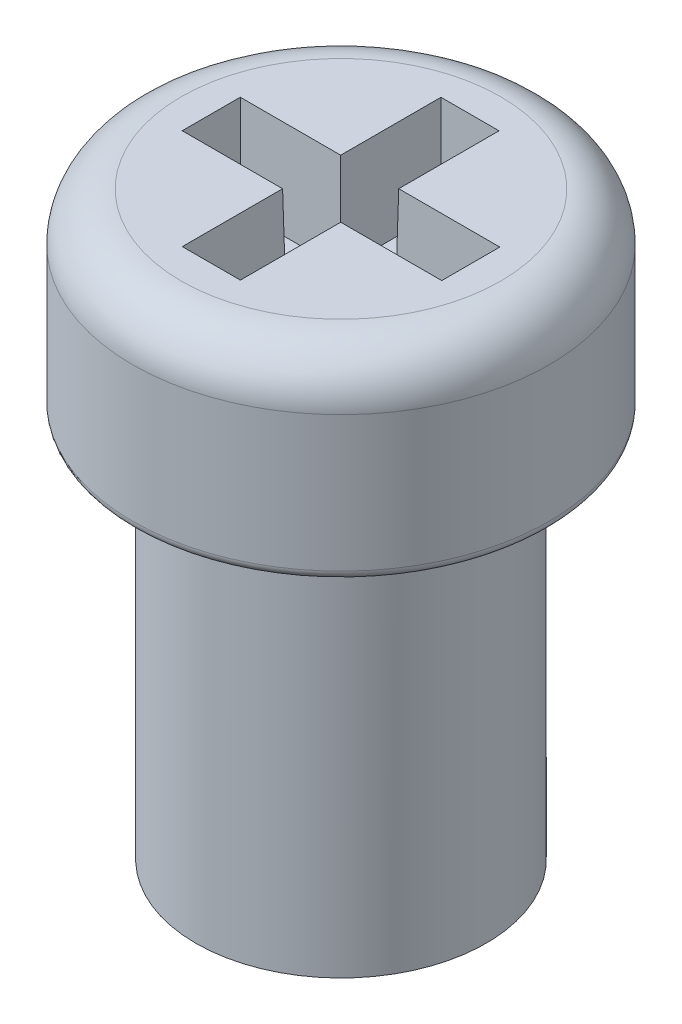
SolidWorks part; units mm, degrees
ref_plane "Front Plane" through (0, 0, 0) normal (0, 0, 1) x (1, 0, 0)
ref_plane "Top Plane" through (0, 0, 0) normal (0, 1, 0) x (1, 0, 0)
ref_plane "Right Plane" through (0, 0, 0) normal (1, 0, 0) x (0, 0, -1)
sketch "Sketch1" plane through (0, 0, 0) normal (0, 1, 0) x (1, 0, 0)
  circle A0 centre (0, 0) radius 2.15
  dimension "D1" = 4.3
extrude "Boss-Extrude1" add sketch "Sketch1" along normal blind 2
sketch "Sketch2" plane through (0, 0, 0) normal (0, -1, 0) x (1, 0, 0)
  circle A0 centre (0, 0) radius 1.5
  dimension "D1" = 3
extrude "Boss-Extrude2" add sketch "Sketch2" along normal blind 4
fillet "Fillet1" radius 0.5 1 edges at (0, 2, 2.15)
fillet "Fillet2" radius 0.1 1 edges at (0, 0, 2.15)
sketch "Sketch3" plane through (0, 2, 0) normal (0, 1, 0) x (1, 0, 0)
  line L0 (0.2966, 0.3) -> (1.3407, 0.3)
  line L1 (-1.3407, -0.3) -> (-0.3034, -0.3)
  line L2 (-1.3407, -0.3) -> (-1.3407, 0.3)
  line L3 (-1.3407, 0.3) -> (-0.3034, 0.3)
  line L4 (1.3407, -0.3) -> (1.3407, 0.3)
  line L5 (0.2966, 0.3) -> (0.2966, 1.3361)
  line L6 (-1.3472, 0.3015) -> (-1.3407, 0.3) construction
  line L7 (-0.3034, -1.3361) -> (0.2966, -1.3361)
  line L8 (-0.3034, -1.3361) -> (-0.3034, -0.3)
  line L9 (-0.3034, 1.3361) -> (0.2966, 1.3361)
  line L10 (0.2966, -1.3361) -> (0.2966, -0.3)
  line L11 (-0.0036, -0.0008) -> (-0.0033, 0.0007) construction
  line L12 (-0.0033, 0.0007) -> (-0.003, -0.0007) construction
  line L13 (-0.3034, 0.3) -> (-0.3034, 1.3361)
  line L15 (0.2966, -0.3) -> (1.3407, -0.3)
  line L17 (-0.0036, -0.0008) -> (0, 0) construction
  line L18 (-0.0033, 0.0007) -> (0, 0) construction
  point P0 (0, 0)
  point P6 (-0.0033, 0.0007)
  dimension "D1" = 0.6
  dimension "D2" = 0.6
extrude "Cut-Extrude1" cut sketch "Sketch3" against normal blind 1 draft 1
